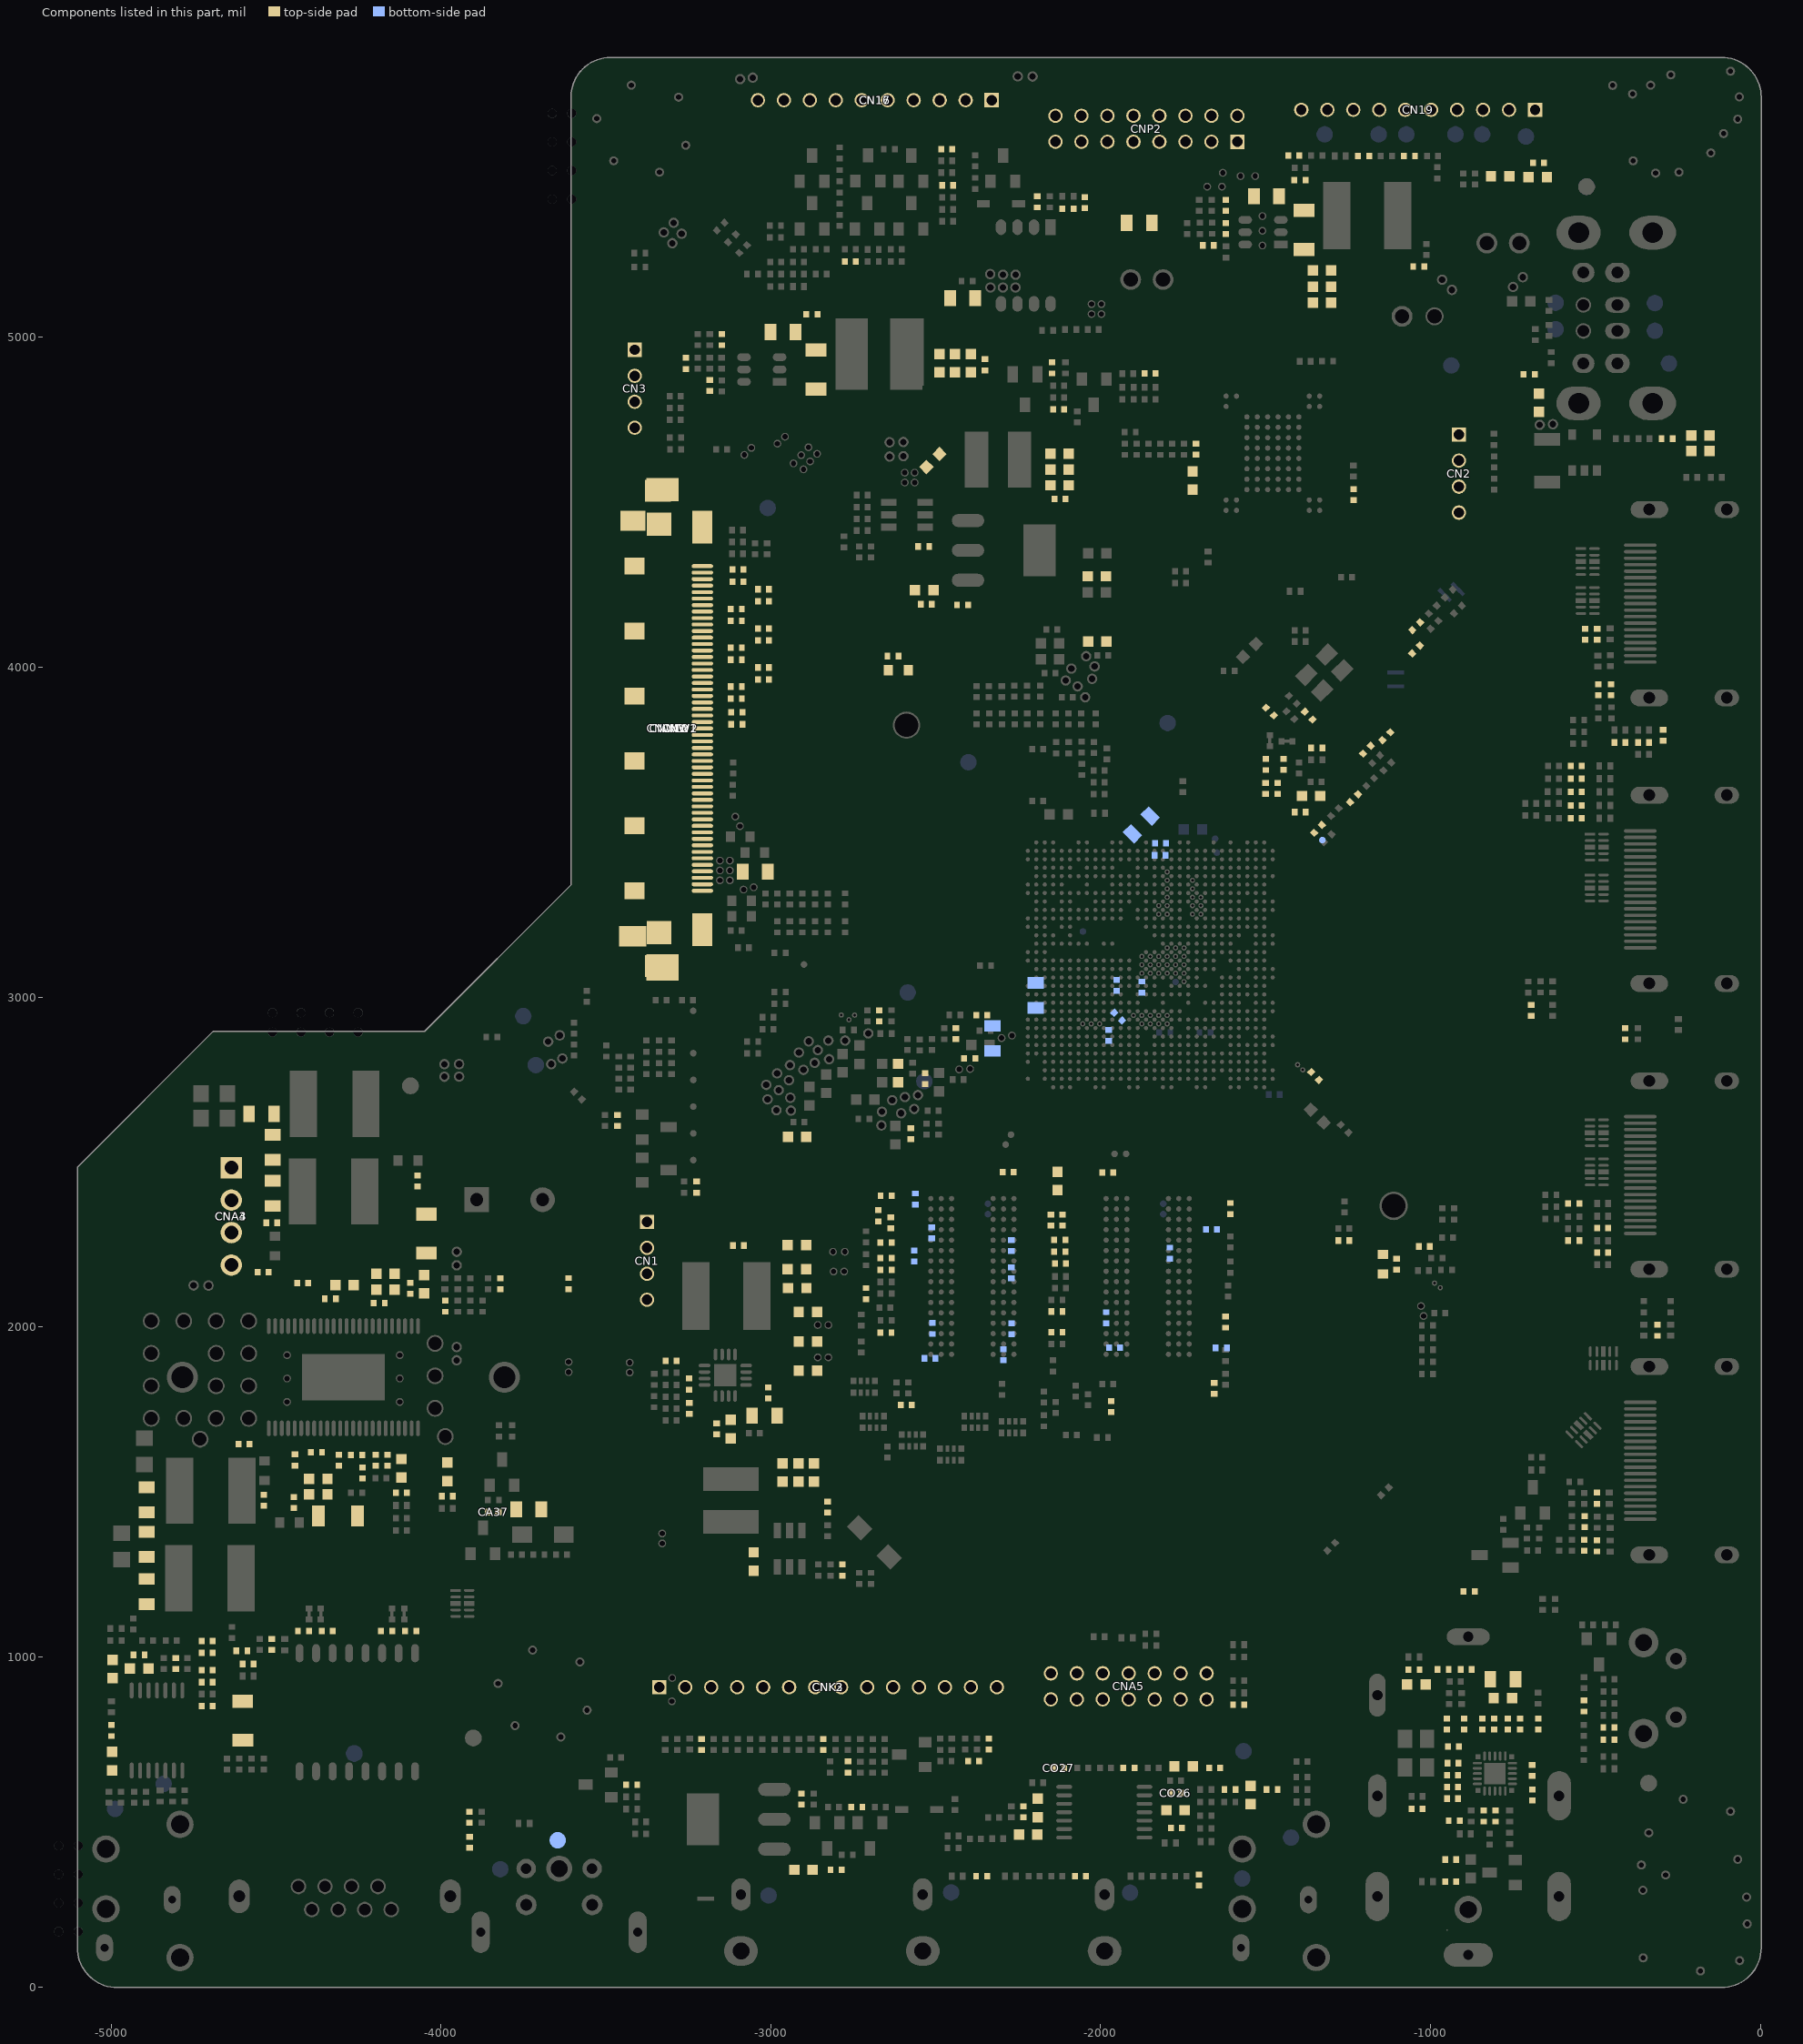
[diagram p0: the components of this part, seen from the top]
# Altium PCB MISC86290.PcbDoc (part 2 of 31)
Units mil, origin at the board's own origin, x right, y up, seen from the top; angles counter-clockwise.
Board outline 5104.71 x 5851.49 mil, 2 copper layers (TopLayer, BottomLayer), stack 61.855 mil thick; 1026 components, 667 nets, 4280 pads, 2294 vias.

## Components (designator, comment, footprint, x,y, rotation, side; value= is the part's Value field where it differs from the comment) (continued)
C51 "Ceramic capacitor,CAP MC,6.3V,10uF,±20%,X5R,0603,SMD,TP" C0603 -2131.01,2442.94 r270 top
C55 "0.047uF-0402-X7R-±10%-16V" C0402#1 -1341,3510 r225 top
C56 "22pF-0402-NPO-±5%-50V" C0402#1 -1486.98,3865.68 r135 top
C57 "22pF-0402-NPO-±5%-50V" C0402#1 -1369.47,3853.53 r315 top
C58 "NC/Ceramic capacitor,CAP MC,16V,0.1uF,±20%,X5R,0402,SMD,TP" C0402#1 -2397,2814.5 r0 top
C59 "Ceramic capacitor,CAP MC,50V,1000pF,±20%,X7R,0402,SMD,TP" C0402#1 -2439.01,2889.4 r90 top
C60 "Ceramic capacitor,CAP MC,16V,0.1uF,±20%,X5R,0402,SMD,TP" C0402#1 -2360.18,2945.53 r180 top
C61 "Ceramic capacitor,CAP MC,6.3V,22uF,±20%,X5R,0603,SMD,TP" C0603 -2887.76,1867.63 r0 top
C62 "Ceramic capacitor,CAP MC,6.3V,22uF,±20%,X5R,0603,SMD,TP" C0603 -2887.76,2045.13 r0 top
C63 "Ceramic capacitor,CAP MC,6.3V,10uF,±20%,X5R,0603,SMD,TP" C0603 -2887.76,1956.38 r0 top
C64 "Ceramic capacitor,CAP MC,6.3V,10uF,±20%,X5R,0603,SMD,TP" C0603 -2614.5,2770 r270 top
C65 "Ceramic capacitor,CAP MC,16V,0.1uF,±20%,X5R,0402,SMD,TP" C0402#1 -2150.88,2323.95 r90 top
C66 "Ceramic capacitor,CAP MC,16V,0.1uF,±20%,X5R,0402,SMD,TP" C0402#1 -2115.35,2323.95 r90 top
C67 "Ceramic capacitor,CAP MC,16V,0.1uF,±20%,X5R,0402,SMD,TP" C0402#1 -1978.98,2468.11 r180 top
C68 "Ceramic capacitor,CAP MC,16V,0.1uF,±20%,X5R,0402,SMD,TP" C0402#1 -2650.85,2172.83 r0 top
C69 "Ceramic capacitor,CAP MC,16V,0.1uF,±20%,X5R,0402,SMD,TP" C0402#1 -2650.85,2255.51 r0 top
C70 "Ceramic capacitor,CAP MC,16V,0.1uF,±20%,X5R,0402,SMD,TP" C0402#1 -1606.61,2359.17 r90 top
C71 "Ceramic capacitor,CAP MC,16V,0.1uF,±20%,X5R,0402,SMD,TP" C0402#1 -2674.26,2337.13 r90 top
C73 "Ceramic capacitor,CAP MC,16V,0.1uF,±20%,X5R,0402,SMD,TP" C0402#1 -2122.05,2192.52 r0 top
C74 "Ceramic capacitor,CAP MC,16V,0.1uF,±20%,X5R,0402,SMD,TP" C0402#1 -1655.84,1813.9 r90 top
C75 "Ceramic capacitor,CAP MC,16V,0.1uF,±20%,X5R,0402,SMD,TP" C0402#1 -2650.49,2397.63 r0 top
C76 "Ceramic capacitor,CAP MC,16V,0.1uF,±20%,X5R,0402,SMD,TP" C0402#1 -2280.16,2470.08 r180 top
C77 "Ceramic capacitor,CAP MC,16V,0.1uF,±20%,X5R,0402,SMD,TP" C0402#1 -2575.5,2585.73 r90 top
C78 "Ceramic capacitor,CAP MC,16V,0.1uF,±20%,X5R,0402,SMD,TP" C0402#1 -2532,2753.23 r90 top
C79 "Ceramic capacitor,CAP MC,16V,0.1uF,±20%,X5R,0402,SMD,TP" C0402#1 -2636.26,2316.13 r90 top
C80 "Ceramic capacitor,CAP MC,16V,0.1uF,±20%,X5R,0402,SMD,TP" C0402#1 -2651,1982.5 r180 top
C81 "Ceramic capacitor,CAP MC,16V,0.1uF,±20%,X5R,0402,SMD,TP" C0402#1 -2132.52,1983.86 r180 top
C82 "Ceramic capacitor,CAP MC,16V,0.1uF,±20%,X5R,0402,SMD,TP" C0402#1 -2124.05,2263.78 r0 top
C83 "NC/Ceramic capacitor,CAP MC,16V,0.1uF,±20%,X5R,0402,SMD,TP" C0402#1 -2294.61,1916.26 r90 bottom
C84 "NC/Ceramic capacitor,CAP MC,16V,0.1uF,±20%,X5R,0402,SMD,TP" C0402#1 -2512.26,2285.13 r90 bottom
C85 "NC/Ceramic capacitor,CAP MC,16V,0.1uF,±20%,X5R,0402,SMD,TP" C0402#1 -1664.01,2295.63 r180 bottom
C86 "NC/Ceramic capacitor,CAP MC,16V,0.1uF,±20%,X5R,0402,SMD,TP" C0402#1 -2510,1995.5 r90 bottom
C87 "NC/Ceramic capacitor,CAP MC,16V,0.1uF,±20%,X5R,0402,SMD,TP" C0402#1 -2562,2388 r90 bottom
C88 "NC/Ceramic capacitor,CAP MC,16V,0.1uF,±20%,X5R,0402,SMD,TP" C0402#1 -1634.49,1936.61 r180 bottom
C89 "NC/Ceramic capacitor,CAP MC,16V,0.1uF,±20%,X5R,0402,SMD,TP" C0402#1 -2565.5,2215.5 r90 bottom
C90 "NC/Ceramic capacitor,CAP MC,16V,0.1uF,±20%,X5R,0402,SMD,TP" C0402#1 -1958.28,1937.13 r180 bottom
C91 "NC/Ceramic capacitor,CAP MC,16V,0.1uF,±20%,X5R,0402,SMD,TP" C0402#1 -2269.72,1994.69 r90 bottom
C92 "NC/Ceramic capacitor,CAP MC,16V,0.1uF,±20%,X5R,0402,SMD,TP" C0402#1 -2270.98,2246.65 r90 bottom
C93 "NC/Ceramic capacitor,CAP MC,16V,0.1uF,±20%,X5R,0402,SMD,TP" C0402#1 -2270.98,2163.98 r90 bottom
C94 "NC/Ceramic capacitor,CAP MC,16V,0.1uF,±20%,X5R,0402,SMD,TP" C0402#1 -2517.63,1905.12 r180 bottom
C95 "NC/Ceramic capacitor,CAP MC,16V,0.1uF,±20%,X5R,0402,SMD,TP" C0402#1 -1790.67,2224.02 r270 bottom
C96 "NC/Ceramic capacitor,CAP MC,16V,0.1uF,±20%,X5R,0402,SMD,TP" C0402#1 -1983.58,2028.15 r270 bottom
C97 "Ceramic capacitor,CAP MC,16V,0.1uF,±20%,X5R,0402,SMD,TP" C0402#1 -1967.83,1758.78 r90 top
C98 "Ceramic capacitor,CAP MC,50V,1000pF,±20%,X7R,0402,SMD,TP" C0402#1 -2124.05,2227.95 r0 top
C99 "Ceramic capacitor,CAP MC,50V,1000pF,±20%,X7R,0402,SMD,TP" C0402#1 -1621.38,2014.69 r90 top
C100 "Ceramic capacitor,CAP MC,50V,1000pF,±20%,X7R,0402,SMD,TP" C0402#1 -2132.52,2046.85 r180 top
C101 "Ceramic capacitor,CAP MC,50V,1000pF,±20%,X7R,0402,SMD,TP" C0402#1 -2650.85,2208.55 r0 top
C102 "Ceramic capacitor,CAP MC,16V,0.1uF,±20%,X5R,0402,SMD,TP" C0402#1 -2711.21,2101.3 r90 top
C103 "Ceramic capacitor,CAP MC,16V,0.1uF,±20%,X5R,0402,SMD,TP" C0402#1 -2589.48,1763.38 r180 top
C110 "0.1uF-0402-X5R-±20%-16V" C0402#1 -2671,2943.52 r90 top
C111 "1uF-0402-X5R-±20%-6.3V" C0402#1 -1350.15,2761.15 r135 top
C164 "2200pF-0402-X7R-±10%-50V" C0402#1 -4309.75,1595.81 r270 top
C174 "Ceramic capacitor,CAP MC,50V,330pF,±5%,NPO,0402,SMD,TP" C0402#1 -1263.27,2262 r180 top
C200 "NC/0ohm-0603-±5%-1/10W" R0603 -2613.5,3991.5 r180 top
C201 "NC/PZ1608U121-2R0TF(120ohm-2000mA)" R0603 -1144,2190 r90 top
C202 "NC/?" C0402#1 -2630,4034 r0 top
C205 "NC/?" C0402#1 -1103,2190 r90 top
C206 "NC/0.1uF-0402-X5R-±20%-16V" C0402#1 -1976,2884 r270 bottom
C207 "NC/0.1uF-0402-X5R-±20%-16V" C0402#1 -1947,2941 r135 bottom
C208 "NC/10uF-0805-X5R-±20%-16V" C0805 -2328,2875.06 r90 bottom
C209 "NC/0.1uF-0402-X5R-±20%-16V" C0402#1 -1819,3467 r180 bottom
C210 "NC/0.1uF-0402-X5R-±20%-16V" C0402#1 -1820,3430 r180 bottom
C211 "NC/10uF-0805-X5R-±20%-16V" C0805 -1877,3522 r225 bottom
C212 "NC/0.1uF-0402-X5R-±20%-16V" C0402#1 -1875,3030.5 r270 bottom
C213 "NC/0.1uF-0402-X5R-±20%-16V" C0402#1 -1952,3036 r270 bottom
C214 "NC/10uF-0805-X5R-±20%-16V" C0805 -2197,3005 r270 bottom
C240 "Ceramic capacitor,CAP MC,6.3V,10uF,±20%,X5R,0603,SMD,TP" C0603 -2010.5,4078.5 r180 top
CA1 "NC/Ceramic capacitor,CAP MC,50V,0.1uF,±10%,X7R,0603,SMD,TP" C0603 -4371.74,1492.1 r180 top
CA2 "Ceramic capacitor,CAP MC,50V,1000pF,±20%,X7R,0402,SMD,TP" C0402#1 -4377.41,1619.77 r180 top
CA3 "4700pF-0402-X7R-±10%-50V" C0402#1 -4197.75,1595.81 r270 top
CA4 "NC/Ceramic capacitor,CAP MC,50V,1uF,±10%,X5R,0603,SMD,TP" C0603 -4371.74,1539.41 r180 top
CA5 "0.047uF-0402-X7R-±10%-16V" C0402#1 -4161.75,1595.81 r90 top
CA6 "NC/Ceramic capacitor,CAP MC,50V,0.1uF,±10%,X7R,0603,SMD,TP" C0603 -4292.5,2127.5 r180 top
CA7 "4700pF-0402-X7R-±10%-50V" C0402#1 -4255.75,1611.81 r0 top
CA8 "Ceramic capacitor,CAP MC,50V,1000pF,±20%,X7R,0402,SMD,TP" C0402#1 -4335.5,2085.5 r180 top
CA9 "0.1uF-0402-X7R-±10%-16V" C0402#1 -4093,2117 r270 top
CA10 "10uF-0603-X5R-±20%-6.3V" C0603 -4051,2130 r270 top
CA11 "0.047uF-0402-X7R-±10%-16V" C0402#1 -4237.75,1557.81 r90 top
CA12 "NC/Ceramic capacitor,CAP MC,50V,1uF,±10%,X5R,0603,SMD,TP" C0603 -4168.5,2161 r180 top
CA13 "0.01uF-0402-X7R-±10%-50V" C0402#1 -4442.75,1596.81 r90 top
CA14 "0.68uF-0805-X7R-±10%-25V" C0805 -4892,1198 r270 top
CA15 "0.1uF-0402-X7R-±10%-16V" C0402#1 -4119.75,1497.81 r0 top
CA16 "10uF-0603-X5R-±20%-6.3V" C0603 -4119.75,1571.81 r90 top
CA17 "0.68uF-0805-X7R-±10%-25V" C0805 -4892.03,1476 r90 top
CA18 "0.47uF-0805-X7R-±10%-50V" C0805 -4892,1341 r270 top
CA19 "0.01uF-0402-X7R-±10%-50V" C0402#1 -4597,1645 r0 top
CA20 "0.1uF-0402-X7R-±10%-16V" C0402#1 -3981,1487 r0 top
CA21 "10uF-0603-X5R-±20%-6.3V" C0603 -3981,1560.81 r90 top
CA22 "0.01uF-0402-X7R-±10%-50V" C0402#1 -4538.77,2166.01 r0 top
CA23 "0.1uF-0402-X7R-±10%-16V" C0402#1 -4187,2072 r0 top
CA24 "0.47uF-0805-X7R-±10%-50V" C0805 -4510.36,2545.01 r90 top
CA25 "Ceramic capacitor,CAP MC,50V,1uF,±10%,X5R,0603,SMD,TP" C0603 -4168.5,2113 r0 top
CA26 "0.68uF-0805-X7R-±10%-25V" C0805 -4510.33,2405.01 r270 top
CA27 "0.68uF-0805-X7R-±10%-25V" C0805 -4544,2646.5 r180 top
CA28 "0.01uF-0402-X7R-±10%-50V" C0402#1 -4419,2133 r180 top
CA29 "NC/Ceramic capacitor,CAP MC,50V,1000pF,±10%,X7R,0402,SMD,TP" C0402#1 -1582,855 r0 top
CA30 "Ceramic capacitor,CAP MC,16V,10uF,±10%,X5R,1206,SMD,TP" C1206 -4044,2283 r90 top
CA31 "Ceramic capacitor,CAP MC,16V,10uF,±10%,X5R,1206,SMD,TP" C1206 -4312.39,1427.52 r180 top
CA32 "NC/330pF-0402-NPO-±5%-50V" C0402#1 -4446.39,1467.52 r90 top
CA33 "NC/330pF-0402-NPO-±5%-50V" C0402#1 -4537.39,1474.52 r270 top
CA34 "NC/330pF-0402-NPO-±5%-50V" C0402#1 -4512.77,2316.01 r180 top
CA35 "NC/330pF-0402-NPO-±5%-50V" C0402#1 -4071,2443 r270 top
CA36 "10uF-0805-X5R-±20%-16V" C0805 -3734,1447 r180 top
CA37 "NC/NC/" C0402#2 -3841,1439 r0 top
CA38 "NC/?" C0402#1 -3987,2063 r270 top
CA39 "NC/?" C0402#1 -3820.35,2131.03 r90 top
CA53 "NC/NC/220pF-0402-NPO-±5%-50V" C0402#1 -4803.84,980 r270 top
CA56 "NC/NC/220pF-0402-NPO-±5%-50V" C0402#1 -4708.52,851 r180 top
CD1 "NC/10uF-1206-X5R-±10%-16V" C1206 -1383.2,5325.94 r90 top
CD2 "NC/1uF-0402-X5R-±20%-16V" C0402#1 -1396,5477 r180 top
CD3 "10uF-0805-X5R-±20%-16V" C0805 -1497.25,5428 r180 top
CD4 "NC/0.1uF-0402-X7R-±10%-16V" C0402#1 -1621.02,5330 r270 top
CD5 "0.1uF-0402-X5R-±20%-16V" C0402#1 -1674,5279 r180 top
CD6 "NC/8pF-0402-NPO-±5%-50V" C0402#1 -1621.25,5400 r270 top
CD7 "NC/0.1uF-0402-X5R-±20%-16V" C0402#1 -1036,5215 r180 top
CD8 "NC/Ceramic capacitor,CAP MC,6.3V,10uF,±20%,X5R,0603,SMD,TP" C0603 -1329.06,5203.75 r0 top
CD9 "NC/Ceramic capacitor,CAP MC,6.3V,10uF,±20%,X5R,0603,SMD,TP" C0603 -1329.06,5153.75 r0 top
CD10 "Ceramic capacitor,CAP MC,6.3V,10uF,±20%,X5R,0603,SMD,TP" C0603 -1329.06,5105.75 r0 top
CD11 "10uF-0805-X5R-±20%-16V" C0805 -2963.28,5016 r180 top
CD12 "NC/0.1uF-0402-X5R-±20%-16V" C0402#1 -2875.5,5070.5 r0 top
CD13 "NC/10uF-1206-X5R-±10%-16V" C1206 -2862.84,4902.69 r90 top
CD14 "0.1uF-0402-X5R-±20%-16V" C0402#1 -3185.25,4854 r90 top
CD15 "NC/8pF-0402-NPO-±5%-50V" C0402#1 -3257.25,4921.27 r270 top
CD16 "NC/0.1uF-0402-X5R-±20%-16V" C0402#1 -2350.75,4917 r90 top
CD17 "Ceramic capacitor,CAP MC,6.3V,10uF,±20%,X5R,0603,SMD,TP" C0603 -2441.75,4922 r90 top
CD18 "Ceramic capacitor,CAP MC,6.3V,10uF,±20%,X5R,0603,SMD,TP" C0603 -2393.75,4922 r90 top
CD19 "Ceramic capacitor,CAP MC,6.3V,10uF,±20%,X5R,0603,SMD,TP" C0603 -2488.75,4922.19 r90 top
CD21 "Ceramic capacitor,CAP MC,6.3V,10uF,±20%,X5R,0603,SMD,TP" C0603 -3052,1289 r270 top
CD22 "0.1uF-0402-X7R-±10%-16V" C0402#1 -2828,1454 r90 top
CD23 "Ceramic capacitor,CAP MC,50V,18pF,±5%,NPO,0402,SMD,TP" C0402#1 -2783.25,1263 r90 top
CD25 "Ceramic capacitor,CAP MC,6.3V,10uF,±20%,X5R,0603,SMD,TP" C0603 -2963.9,1558.87 r90 top
CD26 "Ceramic capacitor,CAP MC,6.3V,10uF,±20%,X5R,0603,SMD,TP" C0603 -2916.59,1558.87 r90 top
CD27 "Ceramic capacitor,CAP MC,6.3V,22uF,±20%,X5R,0603,SMD,TP" C0603 -2869.29,1558.87 r90 top
CD29 "0.1uF-0402-X7R-±10%-16V" C0402#1 -3149,4993 r90 top
CD30 "1uF-0402-X5R-±20%-6.3V" C0402#1 -3007.5,1800.5 r270 top
CD32 "0.1uF-0402-X5R-±20%-16V" C0402#1 -3164.25,1691.27 r90 top
CD33 "NC/10uF-0805-X5R-±20%-16V" C0805 -3019,1731.23 r0 top
CD34 "0.01uF-0402-X7R-±10%-50V" C0402#1 -3247.25,1753 r90 top
CD35 "0.01uF-0402-X7R-±10%-50V" C0402#1 -3248.25,1827 r90 top
CD36 "18pF-0402-NPO-±5%-50V" C0402#1 -3302.5,1897 r180 top
CD38 "Ceramic capacitor,CAP MC,6.3V,10uF,±20%,X5R,0603,SMD,TP" C0603 -2921,2174.75 r180 top
CD39 "0.1uF-0402-X5R-±20%-16V" C0402#1 -3098.25,2247 r0 top
CD40 "Ceramic capacitor,CAP MC,6.3V,10uF,±20%,X5R,0603,SMD,TP" C0603 -2920.5,2577 r180 top
CD41 "Ceramic capacitor,CAP MC,6.3V,10uF,±20%,X5R,0603,SMD,TP" C0603 -2921,2248 r180 top
CD42 "Ceramic capacitor,CAP MC,6.3V,10uF,±20%,X5R,0603,SMD,TP" C0603 -2920,2118 r180 top
CD43 "Ceramic capacitor,CAP MC,6.3V,10uF,±20%,X5R,0603,SMD,TP" C0603 -3121.56,1690.51 r90 top
CD51 "Ceramic capacitor,CAP MC,6.3V,10uF,±20%,X5R,0603,SMD,TP" C0603 -2508.5,4627 r225 top
CD52 "1uF-0402-X5R-±20%-6.3V" C0402#1 -2536.5,4366.23 r180 top
CD53 "Ceramic capacitor,CAP MC,50V,18pF,±5%,NPO,0402,SMD,TP" C0402#1 -2123.7,4509.93 r0 top
CD54 "Ceramic capacitor,CAP MC,6.3V,10uF,±20%,X5R,0603,SMD,TP" C0603 -2124.45,4647.68 r0 top
CD55 "Ceramic capacitor,CAP MC,6.3V,10uF,±20%,X5R,0603,SMD,TP" C0603 -2124.45,4599.68 r0 top
CD56 "Ceramic capacitor,CAP MC,6.3V,22uF,±20%,X5R,0603,SMD,TP" C0603 -2124.45,4551.68 r0 top
CE1 "NC/7pF-0402-NPO-±5%-50V" C0402#1 -4091.77,1078.77 r180 top
CE2 "NC/7pF-0402-NPO-±5%-50V" C0402#1 -4164.73,1078.79 r0 top
CE3 "NC/7pF-0402-NPO-±5%-50V" C0402#1 -4344.77,1078.77 r180 top
CE4 "NC/7pF-0402-NPO-±5%-50V" C0402#1 -4417,1078.79 r0 top
CE5 "1000pF-1206-X7R-±20%-2000V" C1206 -4601,806.5 r90 top
CE6 "0.1uF-0402-X5R-±20%-16V" C0402#1 -4513.06,1037.98 r90 top
CE7 "0.1uF-0402-X5R-±20%-16V" C0402#1 -4603.5,1018.5 r0 top
CE8 "NC/0.01uF-0402-X7R-±10%-16V" C0402#1 -4584.27,978.37 r0 top
CF1 "0.01uF-0402-X7R-±10%-50V" C0402#1 -1711,4661 r270 top
CF2 "0.01uF-0402-X7R-±10%-50V" C0402#1 -1233,4523.5 r90 top
CF3 "Ceramic capacitor,CAP MC,6.3V,10uF,±20%,X5R,0603,SMD,TP" C0603 -1721.5,4566 r90 top
CG1 "NC/1uF-0402-X5R-±20%-6.3V" C0402#1 -2464,5461 r0 top
CG11 "NC/1uF-0402-X5R-±20%-6.3V" C0402#1 -2467,5570.5 r180 top
CG30 "NC/1uF-0402-X5R-±20%-6.3V" C0402#1 -2759,5230 r0 top
CH1 "220pF-0402-NPO-±5%-50V" C0402#1 -354,3772 r0 top
CH2 "NC/22pF-0402-NPO-±5%-50V" C0402#1 -426.27,3772 r0 top
CH4 "NC/22pF-0402-NPO-±5%-50V" C0402#1 -453,3932 r90 top
CH5 "NC/22pF-0402-NPO-±5%-50V" C0402#1 -491,3932 r90 top
CH6 "22pF-0402-NPO-±5%-50V" C0402#1 -495,4100 r270 top
CH7 "1uF-0402-X5R-±20%-6.3V" C0402#1 -531,4100 r270 top
CH11 "220pF-0402-NPO-±5%-50V" C0402#1 -558,3701.01 r0 top
CH12 "220pF-0402-NPO-±5%-50V" C0402#1 -558,3662.01 r0 top
CH13 "NC/22pF-0402-NPO-±5%-50V" C0402#1 -558,3621.99 r0 top
CH14 "NC/22pF-0402-NPO-±5%-50V" C0402#1 -558,3581.01 r0 top
CH15 "22pF-0402-NPO-±5%-50V" C0402#1 -312,1990 r90 top
CH16 "22pF-0402-NPO-±5%-50V" C0402#1 -295,3794 r90 top
CH17 "22pF-0402-NPO-±5%-50V" C0402#1 -558,3541.99 r180 top
CH18 "22pF-0402-NPO-±5%-50V" C0402#1 -410,2889 r90 top
CH21 "220pF-0402-NPO-±5%-50V" C0402#1 -566,2262 r0 top
CH22 "220pF-0402-NPO-±5%-50V" C0402#1 -478,2226 r180 top
CH23 "NC/22pF-0402-NPO-±5%-50V" C0402#1 -478,2300 r180 top
CH24 "NC/22pF-0402-NPO-±5%-50V" C0402#1 -566,2374 r0 top
CH31 "220pF-0402-NPO-±5%-50V" C0402#1 -496,1336.27 r270 top
CH32 "220pF-0402-NPO-±5%-50V" C0402#1 -534,1338 r90 top
CH33 "NC/22pF-0402-NPO-±5%-50V" C0402#1 -533,1410 r270 top
CH34 "NC/22pF-0402-NPO-±5%-50V" C0402#1 -496,1481 r270 top
CI1 "NC/56pF-0402-NPO-±5%-50V" C0402#1 -2361,334.99 r180 top
CI2 "0.047uF-0402-X7R-±10%-16V" C0402#1 -1232,3603 r225 top
CI3 "NC/56pF-0402-NPO-±5%-50V" C0402#1 -2061.27,334.99 r180 top
CI4 "2.2uF-0402-X5R-±20%-6.3V" C0402#1 -1134,3791 r225 top
CI5 "NC/56pF-0402-NPO-±5%-50V" C0402#1 -1702,323 r90 top
CI6 "2.2uF-0402-X5R-±20%-6.3V" C0402#1 -1193,3750 r225 top
CK1 "NC/22pF-0402-NPO-±5%-50V" C0402#1 -2766,666 r90 top
CK3 "0.01uF-0402-X7R-±10%-50V" C0402#1 -3209.91,734.27 r270 top
CK7 "NC/1000pF-0402-X7R-±10%-50V" C0402#1 -2339,735.5 r90 top
CK8 "Ceramic capacitor,CAP MC,50V,1000pF,±20%,X7R,0402,SMD,TP" C0402#1 -2385,684 r180 top
CK9 "0.01uF-0402-X7R-±10%-50V" C0402#1 -2840.75,734.27 r270 top
CL1 "0.1uF-0402-X5R-±20%-16V" C0402#1 -2907.25,569 r270 top
CL2 "Ceramic capacitor,CAP MC,6.3V,10uF,±20%,X5R,0603,SMD,TP" C0603 -2901.25,354.33 r0 top
CL3 "NC/0.1uF-0402-X5R-±20%-16V" C0402#1 -2802.25,354.33 r0 top
CL13 "Ceramic capacitor,CAP MC,6.3V,10uF,±20%,X5R,0603,SMD,TP" C0603 -2535,4234 r0 top
CL25 "NC/0.1uF-0402-X5R-±20%-16V" C0402#1 -2529,4191 r0 top
CL55 "0.1uF-0402-X5R-±20%-16V" C0402#1 -2419,4189.11 r0 top
CM1 "1uF-0402-X5R-±20%-6.3V" C0402#1 -1850.06,4891 r180 top
CM2 "0.022uF-0402-X7R-±10%-16V" C0402#1 -2127.5,4781.5 r180 top
CM3 "22uF-0603-X5R-±20%-6.3V" C0603 -2012.02,4275.9 r180 top
CM4 "0.022uF-0402-X7R-±10%-16V" C0402#1 -2147,4907.54 r90 top
CM15 "NC/0.1uF-0402-X5R-±20%-16V" C0402#1 -2099.25,5390 r0 top
CM16 "0.022uF-0402-X7R-±10%-16V" C0402#1 -2192.25,5411 r90 top
CM17 "NC/10uF-0805-X5R-±20%-16V" C0805 -2418.25,5119 r180 top
CM18 "NC/10uF-0805-X5R-±20%-16V" C0805 -3047,3380.5 r0 top
CN1 "Connector socket,connect jack,4Pin,D2.0,D,Beige,L=2.8mm,DIP,W2011-04SVA-SN8-ENSY,XYDT" SIP4/2.0D-1 -3375.25,2200.63 r270 top
CN2 "Connector socket,connect jack,4Pin,D2.0,D,Beige,L=2.8mm,DIP,W2011-04SVA-SN8-ENSY,XYDT" SIP4/2.0D-1 -914,4587 r270 top
CN3 "Connector socket,connect jack,4Pin,D2.0,D,Beige,L=2.8mm,DIP,W2011-04SVA-SN8-ENSY,XYDT" SIP4/2.0D-1 -3412.5,4844.5 r270 top
CN16 "NC/Connector socket,connect jack,10Pin,D2.0,D,Nature,L=2.8mm,DIP,W2011-10SVA-SN9-ENSY,XYDT" SIP10/2.0D-1 -2685,5719.46 r180 top locked
CN17 "Connector socket,connect jack,10Pin,D2.0,D,SNAP,Nature,L=2.8mm,DIP,W2015-10SVA-BNSY,XYDT" SIP10/2.0D-4 -2685,5719.46 r180 top locked
CN19 "Connector socket,connect jack,10Pin,D2.0,D,SNAP,Nature,L=2.8mm,DIP,W2015-10SVA-BNSY,XYDT" SIP10/2.0D-4 -1037.56,5690.24 r180 top locked
CNA3 "NC/Connector socket,connect jack,4Pin,D2.50,L,STEP,Beige,L=2.8mm,DIP,CNJST" SIP4H/2.5D-4 -4635.54,2335.44 r270 top locked
CNA4 "Connector socket,connect jack,4PIN,D2.50,L,SNAP,STEP,Fool-proofing,Nature,L=3.0mm,DIP,AMA" SIP4H/2.5D-7 -4642.62,2335.44 r270 top
CNA5 "Gold-plated pin,pin connector,2×7Pin,D,D2.0,L=2.6mm,DIP,LD" SIP2*7/2.0D -1915,910.63 r0 top locked
CNK2 "NC/Connector socket,connect jack,14Pin,D2.0,D,Fool-proofing,Nature,L=2.8,DIP,W2011-14SVA-SN9-ENSY,XYDT" SIP14/2.0D-2 -2826.31,908 r0 top
CNK3 "Connector socket,connect jack,14Pin,D2.0,D,SNAP,L=2.8mm,DIP,CNJST" SIP14/2.0D-5 -2826.31,908 r0 top
CNP2 "Connector socket,connect jack,2×8Pin,D2.0,D,SNAP,L=2.6mm,DIP,CNJST" SIP2*8/2.0D-5 -1861.36,5632.37 r180 top locked
CNW1 "NC/FPC socket,FPC connector (B),51Pin,D0.5,Bottom,lock,SMD,78-050251019,DEREN" FFC51H/0.5S-10 -3275.24,3814.53 r270 top locked
CNW2 "FFC socket,FFC connector,51pin,D0.5,SMD,196182-51041-3,P-TWO" FFC51-H/0.5S-1 -3269.08,3814.53 r270 top locked
CNW3 "NC/FFC socket,FFC connector,51Pin,D0.5,Bottom,lock,SMD,F05035FA51M1WL,CT" FFC51H/0.5S-12 -3318.89,3814.53 r270 top
CNW12 "NC/51PIN-0.5-L-M-G-HSFK" FFC51H/0.5SA-1 -3310.52,3814.53 r270 top locked
CO1 "NC/0.1uF-0402-X5R-±20%-16V" C0402#1 -3913.25,438 r90 top
CO2 "NC/330pF-0402-NPO-±5%-50V" C0402#1 -3914.25,513.27 r270 top
CO3 "33pF-0402-NPO-±5%-50V" C0402#1 -1019.23,2244 r0 top
CO4 "0.1uF-0402-X5R-±20%-16V" C0402#1 -1395.27,3561 r0 top
CO5 "Ceramic capacitor,CAP MC,6.3V,10uF,±20%,X5R,0603,SMD,TP" C0603 -1362,3610 r0 top
CO11 "NC/1000pF-0402-X7R-±10%-50V" C0402#1 -1654.77,663.02 r0 top
CO12 "NC/000pF-0402-X7R-±10%-50V" C0402#1 -1480.27,597.85 r180 top
CO13 "Ceramic capacitor,CAP MC,6.3V,10uF,±20%,X5R,0603,SMD,TP" C0603 -1748.69,668.5 r0 top
CO14 "Ceramic capacitor,CAP MC,6.3V,10uF,±20%,X5R,0603,SMD,TP" C0603 -1545.5,581 r90 top
CO15 "Ceramic capacitor,CAP MC,50V,680pF,±5%,NPO,0402,SMD,TP,Walsin" C0402#1 -1914.5,663 r180 top
CO16 "Ceramic capacitor,CAP MC,50V,680pF,±5%,NPO,0402,SMD,TP,Walsin" C0402#1 -1608.27,597.85 r180 top
CO17 "10uF-0603-X5R-±20%-6.3V" C0603 -2191,542 r90 top
CO18 "0.1uF-0402-X5R-±20%-16V" C0402#1 -2234,530 r90 top
CO19 "10uF-0603-X5R-±20%-6.3V" C0603 -2220,461 r180 top
CO20 "10uF-0603-X5R-±20%-6.3V" C0603 -1773,535 r0 top
CO21 "0.1uF-0402-X5R-±20%-16V" C0402#1 -1770,481 r0 top
CO24 "NC/0.1uF-0402-X5R-±20%-16V" C0402#1 -3613,2131.5 r90 top
CO25 "1uF-0402-X5R-±20%-6.3V" C0402#1 -3421.78,612.5 r180 top
CO26 "Ceramic capacitor,CAP MC,50V,100pF,±5%,NPO,0402,SMD,TP" C0402#3 -1773,587 r180 top
CO27 "Ceramic capacitor,CAP MC,50V,100pF,±5%,NPO,0402,SMD,TP" C0402#3 -2127,663 r0 top
CO31 "Ceramic capacitor,CAP MC,50V,1000pF,±20%,X7R,0402,SMD,TP" C0402#1 -4708.52,1048 r0 top
CO32 "Ceramic capacitor,CAP MC,50V,1000pF,±20%,X7R,0402,SMD,TP" C0402#1 -4708.52,959.49 r180 top
CO33 "Ceramic capacitor,CAP MC,6.3V,1uF,±20%,X5R,0402,SMD,TP" C0402#1 -4708.52,1011.82 r180 top
CO34 "Ceramic capacitor,CAP MC,6.3V,1uF,±20%,X5R,0402,SMD,TP" C0402#1 -4708.52,923.34 r0 top
CO35 "10uF-0603-X5R-±20%-6.3V" C0603 -4995,963 r270 top
CO36 "10uF-0603-X5R-±20%-6.3V" C0603 -4997,684 r270 top
CO37 "0.1uF-0402-X5R-±20%-16V" C0402#1 -4999,776.5 r90 top
CO41 "10uF-0603-X5R-±20%-6.3V" C0603 -4915,964 r0 top
CO42 "0.1uF-0402-X5R-±20%-16V" C0402#1 -4915,1006 r0 top
CO51 "Ceramic capacitor,CAP MC,50V,1000pF,±20%,X7R,0402,SMD,TP" C0402#1 -1043.57,4124.61 r45 top
CO52 "Ceramic capacitor,CAP MC,50V,1000pF,±20%,X7R,0402,SMD,TP" C0402#1 -1044,4054 r45 top
COAX "TEST" TP -3646.25,444 r180 bottom
CP1 "10uF-0805-X5R-±20%-16V" C0805 -1883,5347 r180 top
CP2 "NC/0.1uF-0402-X5R-±20%-16V" C0402#1 -2048,5409 r270 top
CQC "CQC" CQC -2766,3543.2 r0 top
CR1 "1uF-0402-X5R-±20%-6.3V" C0402#1 -459.5,785.5 r0 top
CR2 "0.1uF-0402-X5R-±20%-16V" C0402#1 -883,1198 r0 top
CR3 "0.1uF-0402-X5R-±20%-16V" C0402#1 -535,851 r90 top
CR4 "0.1uF-0402-X5R-±20%-16V" C0402#1 -459.5,748.5 r180 top
CR5 "0.01uF-0402-X7R-±10%-50V" C0402#1 -2739.25,545 r0 top
CT1 "Ceramic capacitor,CAP MC,50V,1000pF,±20%,X7R,0402,SMD,TP" C0402#1 -933.03,570.15 r0 top
CT2 "Ceramic capacitor,CAP MC,50V,1000pF,±20%,X7R,0402,SMD,TP" C0402#1 -928.36,503.15 r0 top
CT3 "10uF-0603-X5R-±20%-6.3V" C0603 -1043,916 r180 top
CT4 "22pF-0402-NPO-±5%-50V" C0402#1 -691,581.5 r270 top
CT5 "22pF-0402-NPO-±5%-50V" C0402#1 -692,655.5 r90 top
CT6 "NC/47pF-0402-NPO-±5%-50V" C0402#1 -961.82,961.61 r0 top
CT7 "33pF-0402-NPO-±5%-50V" C0402#1 -950.82,796.61 r90 top
CT8 "33pF-0402-NPO-±5%-50V" C0402#1 -897.82,796.61 r270 top
CT9 "30pF-0402-NPO-±5%-50V" C0402#1 -802.89,517.37 r270 top
CT10 "0.1uF-0402-X5R-±20%-16V" C0402#1 -673,796 r90 top
CT12 "NC/47pF-0402-NPO-±5%-50V" C0402#1 -1445.5,3706 r90 top
CT13 "0.022uF-0402-X7R-±10%-16V" C0402#1 -1345,3755.5 r0 top
CT14 "NC/47pF-0402-NPO-±5%-50V" C0402#1 -1499.5,3705.23 r90 top
CT15 "1uF-0402-X5R-±20%-6.3V" C0402#1 -933.03,605.15 r180 top
CT16 "1uF-0402-X5R-±20%-6.3V" C0402#1 -766.03,796.5 r270 top
CT17 "Ceramic capacitor,CAP MC,50V,1000pF,±20%,X7R,0402,SMD,TP" C0402#1 -728.39,796.1 r270 top
CT19 "Ceramic capacitor,CAP MC,50V,1000pF,±20%,X7R,0402,SMD,TP" C0402#1 -933.03,641.15 r0 top
CT20 "Ceramic capacitor,CAP MC,50V,1000pF,±20%,X7R,0402,SMD,TP" C0402#1 -806.82,796.61 r270 top
CT21 "NC/47pF-0402-NPO-±5%-50V" C0402#1 -891.82,961.61 r0 top
CT23 "30pF-0402-NPO-±5%-50V" C0402#1 -838.89,517.37 r270 top
CT24 "NC/180pF-0402-NPO-±5%-50V" C0402#1 -938.7,385.3 r180 top
CT25 "Ceramic capacitor,CAP MC,50V,1000pF,±20%,X7R,0402,SMD,TP" C0402#1 -938.7,318.3 r0 top
CT26 "22pF-0402-NPO-±5%-50V" C0402#1 -1041,539 r0 top
CT27 "0.1uF-0402-X5R-±20%-16V" C0402#1 -1464,3632.48 r90 top
CT28 "NC/0.1uF-0805-X7R-±10%-50V" C0805 -780.79,932.61 r180 top
CT30 "10uF-0603-X5R-±20%-6.3V" C0603 -780.82,874.61 r180 top
CT31 "1uF-0402-X5R-±20%-6.3V" C0402#1 -842.82,796.61 r270 top
CT32 "0.1uF-0402-X5R-±20%-16V" C0402#1 -1500,3632.48 r270 top
CT33 "0.1uF-0402-X5R-±20%-16V" C0402#1 -1050,961 r180 top
CT39 "Ceramic capacitor,CAP MC,50V,12pF,±5%,NPO,0402,SMD,TP" C0402#1 -930.91,728.42 r180 top
CT40 "Ceramic capacitor,CAP MC,50V,12pF,±5%,NPO,0402,SMD,TP" C0402#1 -932.38,677.86 r0 top
CU1 "0.1uF-0402-X5R-±20%-16V" C0402#1 -283,4693 r180 top
CU2 "10uF-0603-X5R-±20%-6.3V" C0603 -182,4656 r0 top
CU3 "NC/10uF-0603-X5R-±20%-6.3V" C0603 -671,4802 r270 top
CU4 "0.1uF-0402-X5R-±20%-16V" C0402#1 -701,4888 r0 top
CU5 "10uF-0603-X5R-±20%-6.3V" C0603 -182,4703 r0 top
CU11 "NC/0.1uF-0402-X5R-±20%-16V" C0402#1 -1415,5551 r180 top
CU12 "NC/0.1uF-0402-X5R-±20%-16V" C0402#1 -1203,5550 r180 top
CU13 "NC/0.1uF-0402-X5R-±20%-16V" C0402#1 -1063.89,5550.24 r180 top
CU14 "0.1uF-0402-X5R-±20%-16V" C0402#1 -673.17,5529 r180 top
CU15 "NC/10uF-0603-X5R-±20%-6.3V" C0603 -789.17,5489 r0 top
CU16 "22uF-0603-X5R-±20%-6.3V" C0603 -675.17,5486 r180 top
CVBSOUT1 "TEST" TP-20#1 -1328,3476 r90 bottom
CW244 "0.1uF-0402-X5R-±20%-16V" C0402#1 -3102.98,3827 r180 top
CW245 "0.1uF-0402-X5R-±20%-16V" C0402#1 -3102.98,3863.46 r180 top
CW246 "0.1uF-0402-X5R-±20%-16V" C0402#1 -3104.52,3905 r180 top
CW247 "0.1uF-0402-X5R-±20%-16V" C0402#1 -3104.52,3941.45 r180 top
CW248 "0.1uF-0402-X5R-±20%-16V" C0402#1 -3022.56,3963.16 r180 top
CW249 "0.1uF-0402-X5R-±20%-16V" C0402#1 -3022.56,3999.61 r180 top
CW250 "0.1uF-0402-X5R-±20%-16V" C0402#1 -3104.52,4022.84 r180 top
CW251 "0.1uF-0402-X5R-±20%-16V" C0402#1 -3104.52,4059.3 r180 top
CW252 "0.1uF-0402-X5R-±20%-16V" C0402#1 -3022.56,4081.16 r180 top
CW253 "0.1uF-0402-X5R-±20%-16V" C0402#1 -3022.56,4117.61 r180 top
CW254 "0.1uF-0402-X5R-±20%-16V" C0402#1 -3104.52,4140.39 r180 top
CW255 "0.1uF-0402-X5R-±20%-16V" C0402#1 -3104.52,4176.84 r180 top
CW256 "0.1uF-0402-X5R-±20%-16V" C0402#1 -3022.56,4200.33 r180 top
CW257 "0.1uF-0402-X5R-±20%-16V" C0402#1 -3022.56,4236.79 r180 top
CW258 "0.1uF-0402-X5R-±20%-16V" C0402#1 -3099.25,4259.84 r180 top
CW259 "0.1uF-0402-X5R-±20%-16V" C0402#1 -3099.25,4296.3 r180 top
D4 "NC/TVS diode,DIO ESD,3pF,58V,0402,SMD,SDV1005H260C030YPTF,Sunlord" DIODE-S0402 -3465,2626 r270 top
D5 "NC/TVS diode,DIO ESD,3pF,58V,0402,SMD,SDV1005H260C030YPTF,Sunlord" DIODE-S0402 -3225,2424 r90 top
D40 "NC/SFI0402-240E-2R5PP-LF" DIODE-S0402 -695,2960 r90 top